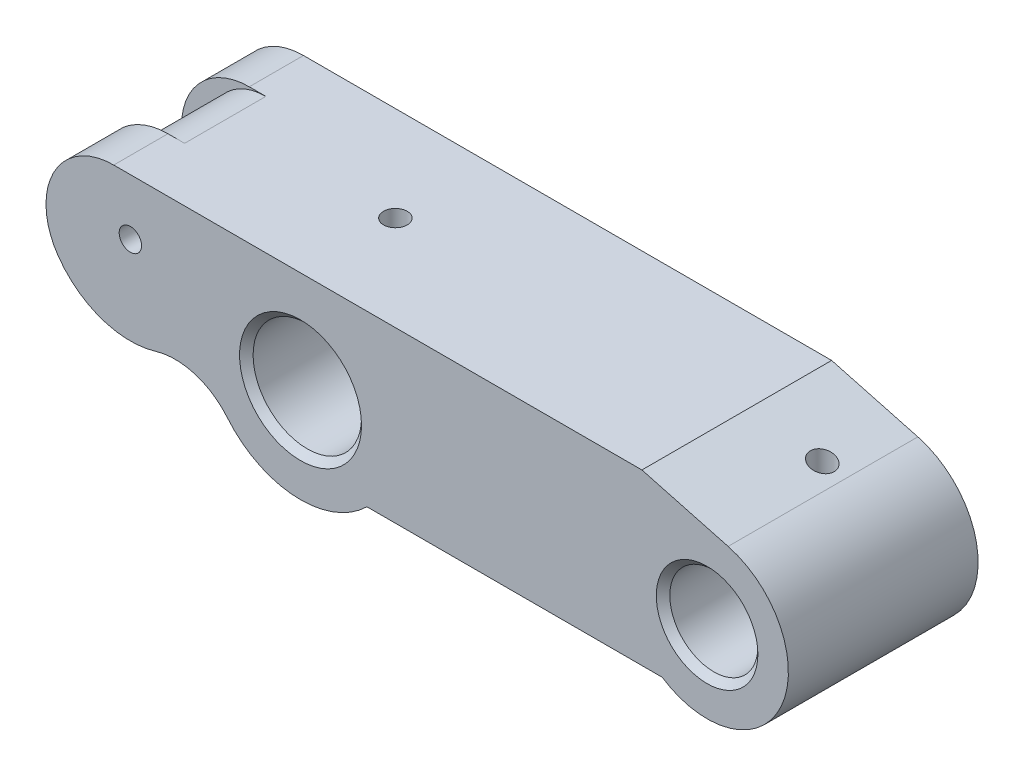
SolidWorks part; units mm, degrees
ref_plane "Front Plane" through (0, 0, 0) normal (0, 0, 1) x (1, 0, 0)
ref_plane "Top Plane" through (0, 0, 0) normal (0, 1, 0) x (1, 0, 0)
ref_plane "Right Plane" through (0, 0, 0) normal (1, 0, 0) x (0, 0, -1)
other "Configuration Table"
sketch "Sketch1" plane through (0, 0, 0) normal (0, 0, 1) x (1, 0, 0)
  line L0 (0, 0) -> (30.1627, 0) construction
  line L1 (0, 0) -> (-25.1141, 6.7293) construction
  line L4 (9.798, -10) -> (53.3668, -10)
  line L5 (-25.1141, 15.0003) -> (50.3826, 15.0003)
  line L6 (50.3826, 15.0003) -> (63.1058, 11.5911)
  circle A0 centre (0, 0) radius 8
  circle A1 centre (60, 0) radius 6.5
  arc A2 (53.3668, -10) -> (63.1058, 11.5911) centre (60, 0) ccw
  arc A3 (-12.4032, -6.4932) -> (9.798, -10) centre (0, 0) ccw
  arc A4 (-25.1141, 15.0003) -> (-23.3706, -1.3559) centre (-25.1141, 6.7293) ccw
  arc A5 (-12.4032, -6.4932) -> (-23.3706, -1.3559) centre (-21.2626, -11.1311) ccw
  circle A6 centre (-25.1141, 6.7293) radius 1.5
  dimension "D1" = 16
  dimension "D2" = 13
  dimension "D4" = 24
  dimension "D5" = 28
  dimension "D8" = 16.542
  dimension "D12" = 10
  dimension "D13" = 3
  dimension "D3" = 60
  dimension "D6" = 26
  dimension "D7" = 15
  dimension "D9" = 10
  dimension "D10" = 25.0003
  dimension "D11" = 15
extrude "Boss-Extrude1" add sketch "Sketch1" along normal mid plane 12
sketch "Sketch2" plane through (0, 0, 6) normal (0, 0, 1) x (1, 0, 0)
  line L1 (63.1058, 11.5911) -> (50.3826, 15.0003) construction
  line L2 (9.798, -10) -> (53.3668, -10) construction
  line L3 (50.3826, 15.0003) -> (-27.5657, 15.0003)
  line L4 (63.1058, 11.5911) -> (50.3826, 15.0003)
  line L5 (9.798, -10) -> (53.3668, -10)
  arc A0 (53.3668, -10) -> (63.1058, 11.5911) centre (60, 0) ccw construction
  arc A2 (53.3668, -10) -> (63.1058, 11.5911) centre (60, 0) ccw
  arc A3 (-10.7877, -8.9233) -> (9.798, -10) centre (0, 0) ccw
  arc A4 (-35.7379, -0.763) -> (-21.3718, -5.7204) centre (-25.1141, 6.7293) ccw
  arc A5 (-10.7877, -8.9233) -> (-21.3718, -5.7204) centre (-18.4932, -15.2971) ccw
  arc A6 (-27.5657, 15.0003) -> (-35.7379, -0.763) centre (-27.5657, 5.0003) ccw
  circle A7 centre (60, 0) radius 6.5 construction
  circle A8 centre (0, 0) radius 8 construction
  circle A9 centre (60, 0) radius 6.5
  circle A10 centre (0, 0) radius 8
  dimension "D1" = 26
  dimension "D2" = 20
  dimension "D3" = 10
extrude "Boss-Extrude2" add sketch "Sketch2" along normal blind 8
mirror "Mirror1" about plane through (0, 0, 0) normal (0, 0, 1) of "Boss-Extrude2"
hole_wizard "M4 Tapped Hole1" positions "3DSketch1" profile "Sketch3" tap size "M4" standard "GB"
sketch3d "3DSketch1"
  point P0 (-25.1141, 6.7293, 14)
sketch "Sketch3" plane through (-25.1141, 6.7293, 14) normal (1, 0, 0) x (0, -1, 0)
  line L0 (0, 0) -> (0, 8.9914)
  line L1 (0, 8.9914) -> (1.65, 8)
  line L2 (1.65, 8) -> (1.65, 0)
  line L5 (1.65, 0) -> (0, 0)
  line L10 (0, 8.9914) -> (-1.65, 8) construction
  line L11 (0, -6.35) -> (0, 107.95) construction
  dimension "螺纹孔钻头直径" = 3.3
  dimension "螺纹孔钻头深度" = 8
  dimension "导头角度" = 118
cosmetic thread "Cosmetic Thread1" parameters "D1"=8, "D2"=4
mirror "Mirror2" about plane through (0, 0, 0) normal (0, 0, 1) of "M4 Tapped Hole1"
sketch "Sketch4" plane through (0, 15.0003, 0) normal (0, 1, 0) x (1, 0, 0)
  circle A0 centre (0, 0) radius 1.75
  dimension "D1" = 3.5
extrude "Cut-Extrude1" cut sketch "Sketch4" against normal up to next contours A0
sketch "Sketch5" plane through (0, 15.0003, 0) normal (0, 1, 0) x (1, 0, 0)
  line L0 (66.5, 14) -> (53.5, 14) construction
  line L1 (66.5, 14) -> (53.5, 14) construction
  line L2 (60, 14) -> (60, 3) construction
  circle A0 centre (60, 3) radius 1.75
  dimension "D1" = 3.5
  dimension "D2" = 11
extrude "Cut-Extrude2" cut sketch "Sketch5" against normal up to next
chamfer "Chamfer1" distance 1 angle 45 4 edges at (8, 0, -14) (66.5, 0, -14) (66.5, 0, 14) (8, 0, 14)
